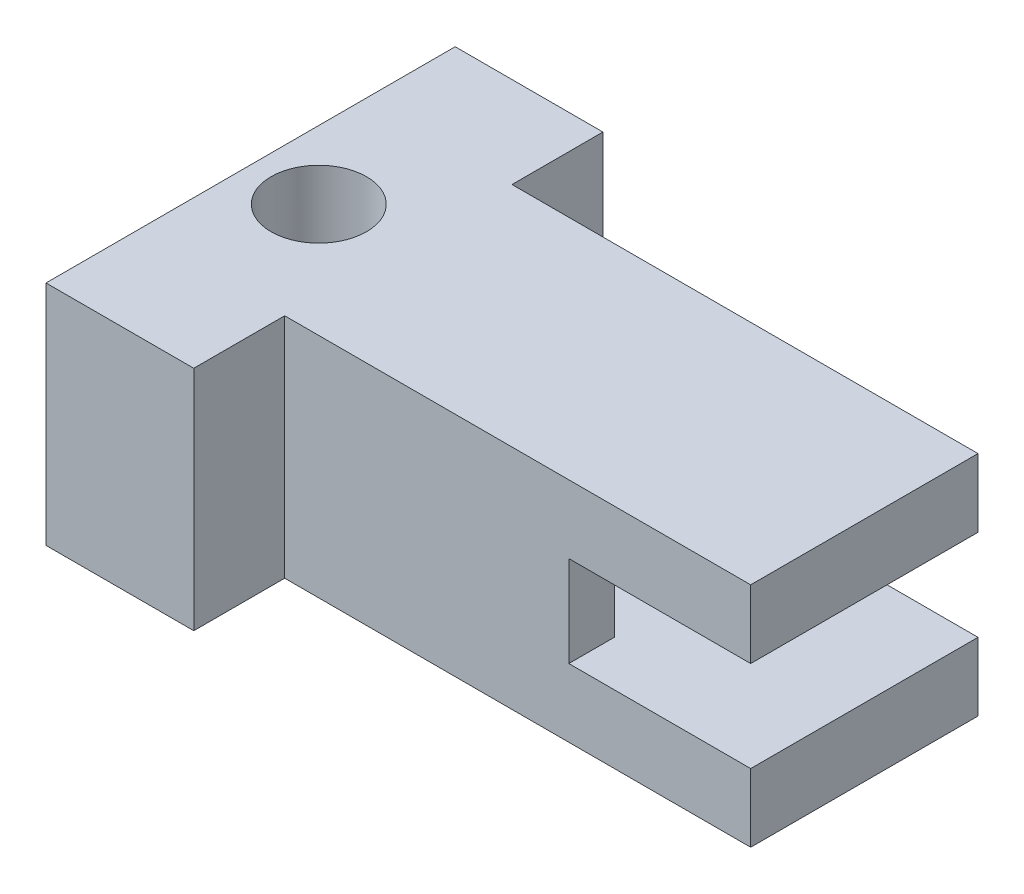
SolidWorks part; units mm, degrees
ref_plane "Front Plane" through (0, 0, 0) normal (0, 0, 1) x (1, 0, 0)
ref_plane "Top Plane" through (0, 0, 0) normal (0, 1, 0) x (1, 0, 0)
ref_plane "Right Plane" through (0, 0, 0) normal (1, 0, 0) x (0, 0, -1)
sketch "Sketch1" plane through (0, 0, 0) normal (0, 1, 0) x (1, 0, 0)
  line L1 (8, -5) -> (-8, -5)
  line L2 (8, -5) -> (8, 5)
  line L3 (8, 5) -> (-8, 5)
  line L4 (-8, -5) -> (-8, 5)
  line L5 (8, -5) -> (-8, 5) construction
  line L6 (8, 5) -> (-8, -5) construction
  point P0 (0, 0)
  dimension "D1" = 10
  dimension "D2" = 16
extrude "Boss-Extrude1" add sketch "Sketch1" along normal blind 10
sketch "Sketch2" plane through (0, 0, -5) normal (0, 0, -1) x (-1, 0, 0)
  line L0 (-8, 10) -> (-8, 0) construction
  line L1 (-16, 3) -> (0, 3)
  line L2 (-16, 3) -> (-16, 7)
  line L3 (-16, 7) -> (0, 7)
  line L4 (0, 3) -> (0, 7)
  line L5 (-16, 3) -> (0, 7) construction
  line L6 (-16, 7) -> (0, 3) construction
  point P0 (-8, 5)
  dimension "D1" = 4
  dimension "D2" = 16
extrude "Cut-Extrude1" cut sketch "Sketch2" against normal blind 10
sketch "Sketch3" plane through (-8, 0, 0) normal (-1, 0, 0) x (0, 0, 1)
  line L1 (-5, 10) -> (5, 10)
  line L2 (-5, 10) -> (-5, 0)
  line L3 (-5, 0) -> (5, 0)
  line L4 (5, 10) -> (5, 0)
extrude "Boss-Extrude2" add sketch "Sketch3" along normal blind 7
sketch "Sketch4" plane through (0, 0, -5) normal (0, 0, -1) x (-1, 0, 0)
  line L0 (-8, 0) -> (15, 0) construction
  line L1 (15, 0) -> (12.5, 0)
  line L2 (15, 0) -> (15, 10)
  line L3 (15, 10) -> (12.5, 10)
  line L4 (12.5, 0) -> (12.5, 10)
  line L5 (-8, 10) -> (15, 10) construction
  line L6 (15, 10) -> (15, 0) construction
  dimension "D1" = 2.5
extrude "Boss-Extrude3" add sketch "Sketch4" along normal blind 4
ref_plane "Plane1" through (0, 0, 0) normal (0, 0, -1) x (-1, 0, 0)
mirror "Mirror1" about plane through (0, 0, 0) normal (0, 0, -1) of "Boss-Extrude3"
sketch "Sketch5" plane through (0, 0, 0) normal (1, 0, 0) x (0, 0, -1)
  line L0 (0, -5.5) -> (0, 5.5) construction
  line L1 (3, 3) -> (-3, 3)
  line L2 (3, 3) -> (3, 7)
  line L3 (3, 7) -> (-3, 7)
  line L4 (-3, 3) -> (-3, 7)
  line L5 (3, 3) -> (-3, 7) construction
  line L6 (3, 7) -> (-3, 3) construction
  line L7 (-5, 7) -> (5, 7) construction
  point P0 (0, 5)
  dimension "D1" = 6
extrude "Cut-Extrude2" cut sketch "Sketch5" against normal blind 4
sketch "Sketch6" plane through (-4, 0, 0) normal (1, 0, 0) x (0, 0, -1)
  line L0 (0, -5.5) -> (0, 5.5) construction
  circle A0 centre (0, 5) radius 1
  dimension "D1" = 2
extrude "Boss-Extrude4" add sketch "Sketch6" along normal blind 3
sketch "Sketch7" plane through (-1, 0, 0) normal (1, 0, 0) x (0, 0, -1)
  circle A0 centre (0, 5) radius 1.3
  dimension "D1" = 2.6
extrude "Boss-Extrude5" add sketch "Sketch7" against normal blind 1
sketch "Sketch8" plane through (-15, 0, 0) normal (-1, 0, 0) x (0, 0, 1)
  line L1 (-9, 10) -> (9, 10)
  line L2 (-9, 10) -> (-9, 0)
  line L3 (-9, 0) -> (9, 0)
  line L4 (9, 10) -> (9, 0)
extrude "Boss-Extrude6" add sketch "Sketch8" along normal blind 4
sketch "Sketch9" plane through (0, 0, 0) normal (0, -1, 0) x (1, 0, 0)
  line L0 (-19, -9) -> (-19, 9) construction
  circle A0 centre (-16, 0) radius 1
  point P0 (-16, 0)
  dimension "D1" = 2
  dimension "D2" = 3
hole_wizard "Tap Drill for M5 Tap1" positions "Sketch9" profile "Sketch10" hole size "M5" standard "GB"
sketch "Sketch10" plane through (-16, 0, 0) normal (1, 0, 0) x (0, 0, -1)
  line L0 (0, 0) -> (0, 61.2618)
  line L1 (0, 61.2618) -> (2.1, 60)
  line L2 (2.1, 60) -> (2.1, 0)
  line L5 (2.1, 0) -> (0, 0)
  line L10 (0, 61.2618) -> (-2.1, 60) construction
  line L11 (0, -6.35) -> (0, 107.95) construction
  dimension "孔直径" = 4.2
  dimension "孔深度" = 60
  dimension "导头角度" = 118
